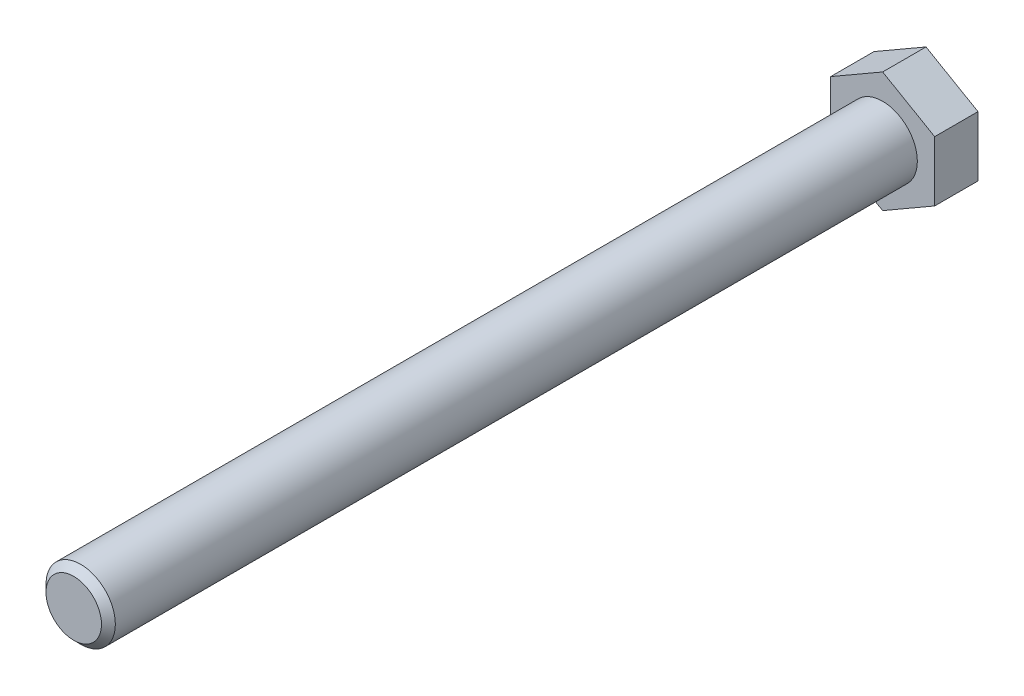
from build123d import *

# Parameters (mm, degrees)
BOSS_EXTRUDE1_DEPTH = 7.5
SKETCH3_R           = 6
BOSS_EXTRUDE2_DEPTH = 140
CHAMFER1_SIZE       = 1.2


with BuildPart() as part:
    # Sketch1 → Boss-Extrude1 (new body)
    with BuildSketch(Plane.XY):
        Polygon((9, 5.196152423), (0, 10.392304845), (-9, 5.196152423), (-9, -5.196152423), (0, -10.392304845), (9, -5.196152423), align=None)
    extrude(amount=BOSS_EXTRUDE1_DEPTH)

    # Sketch3 → Boss-Extrude2 (add)
    with BuildSketch(Plane.XY.offset(7.5)):
        Circle(SKETCH3_R)
    extrude(amount=BOSS_EXTRUDE2_DEPTH)

    # Chamfer1
    chamfer1_edges = [part.edges().sort_by_distance(p)[0] for p in [
        (-6, 0, 147.5),
    ]]
    chamfer(chamfer1_edges, length=CHAMFER1_SIZE)


solid = part.part
